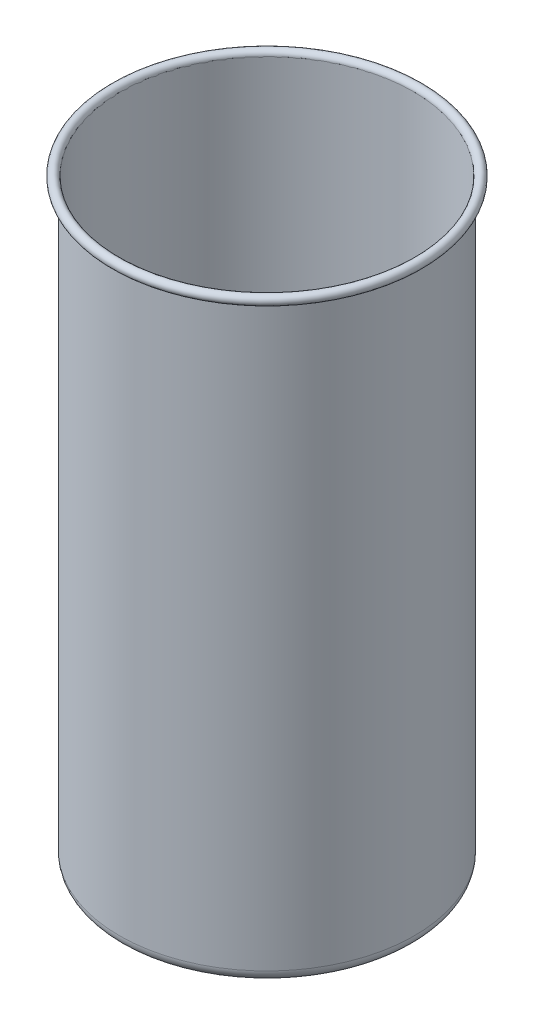
from build123d import *

# Parameters (mm, degrees)
SKETCH1_R           = 125
BOSS_EXTRUDE1_DEPTH = 505
FILLET1_R           = 10
SHELL1_T            = -1
SKETCH6_R           = 4
SKETCH6_R_2         = 3


with BuildPart() as part:
    # Sketch1 → Boss-Extrude1 (new body)
    with BuildSketch(Plane(origin=(0, 0, 0), x_dir=(1, 0, 0), z_dir=(0, 1, 0))):
        with Locations(Location((0, 0, 0), (0, 0, 270))):
            Circle(SKETCH1_R)
    extrude(amount=BOSS_EXTRUDE1_DEPTH)

    # Fillet1
    fillet1_edges = [part.edges().sort_by_distance(p)[0] for p in [
        (0, 0, -125),
    ]]
    fillet(fillet1_edges, radius=FILLET1_R)

    # Shell1
    shell1_openings = [part.faces().sort_by_distance(p)[0] for p in [
        (0, 505, 0),
    ]]
    offset(amount=SHELL1_T, openings=shell1_openings, kind=Kind.INTERSECTION)


with BuildPart() as body_2:
    # Sketch6 → Revolve1 (revolve)
    with BuildSketch(Plane.XY, mode=Mode.PRIVATE) as revolve1_sk:
        with Locations((128, 505)):
            Circle(SKETCH6_R)
        with Locations((128, 505)):
            Circle(SKETCH6_R_2, mode=Mode.SUBTRACT)
    revolve(revolve1_sk.sketch.rotate(Axis((0, 505, 0), (0, 1, 0)), 90), axis=Axis((0, 505, 0), (0, 1, 0)))


solid = Compound([part.part, body_2.part])
